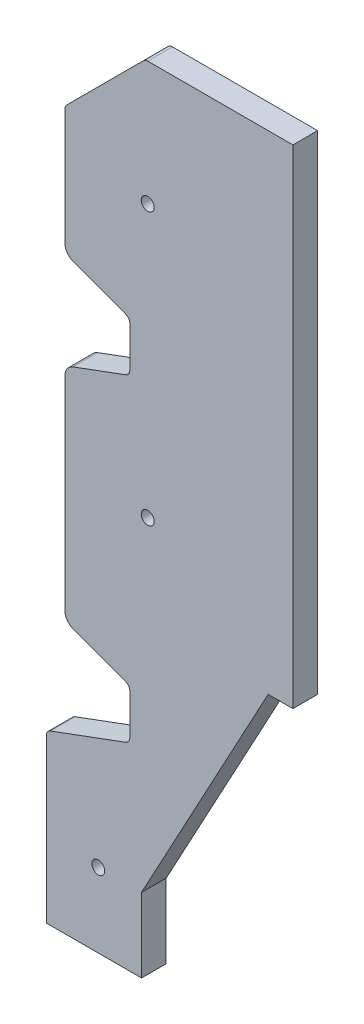
from build123d import *

# Parameters (mm, degrees)
BOSS_EXTRUDE1_DEPTH = 40
CHAMFER1_SIZE       = 160
M24_TAPPED_HOLE1_D  = 21
CUT_EXTRUDE1_DEPTH  = 1351.88896657
FILLET1_R           = 10
SKETCH4_W           = 30
SKETCH4_H           = 822.818816594
CUT_EXTRUDE2_DEPTH  = 1351.88896657
FILLET2_R           = 20
FILLET3_R           = 10


with BuildPart() as part:
    # Sketch1 → Boss-Extrude1 (new body)
    with BuildSketch(Plane.XY):
        Polygon((154, 0), (154, 120), (359, 500), (399, 500), (399, 1290), (0, 1290), (0, 0), align=None)
    extrude(amount=BOSS_EXTRUDE1_DEPTH)

    # Chamfer1
    chamfer1_edges = [part.edges().sort_by_distance(p)[0] for p in [
        (0, 1290, 20),
    ]]
    chamfer(chamfer1_edges, length=CHAMFER1_SIZE)

    # M24 Tapped Hole1 (through all)
    with Locations(Plane(origin=(164, 1090, 0), x_dir=(-1, 0, 0), z_dir=(0, 0, -1))):
        with Locations((0, 0), (0, -440), (80, -970)):
            Hole(M24_TAPPED_HOLE1_D / 2)

    # Sketch3 → Cut-Extrude1 (cut, through all)
    with BuildSketch(Plane(origin=(0, 0, 0), x_dir=(-1, 0, 0), z_dir=(0, 0, -1))):
        Polygon((-135, 835), (0, 785), (0, 965), (-135, 915), align=None)
        Polygon((-135, 400), (-135, 320), (0, 270), (0, 450), align=None)
    extrude(amount=-CUT_EXTRUDE1_DEPTH, mode=Mode.SUBTRACT)

    # Fillet1
    fillet1_edges = [part.edges().sort_by_distance(p)[0] for p in [
        (135, 400, 20),
        (0, 450, 20),
        (0, 270, 20),
        (135, 320, 20),
        (0, 965, 20),
        (0, 785, 20),
        (135, 835, 20),
        (135, 915, 20),
    ]]
    fillet(fillet1_edges, radius=FILLET1_R)

    # Sketch4 → Cut-Extrude2 (cut, through all)
    with BuildSketch(Plane(origin=(0, 0, 0), x_dir=(-1, 0, 0), z_dir=(0, 0, -1))):
        with Locations((-15, 748.590591703)):
            Rectangle(SKETCH4_W, SKETCH4_H)
    extrude(amount=-CUT_EXTRUDE2_DEPTH, mode=Mode.SUBTRACT)

    # Fillet2
    fillet2_edges = [part.edges().sort_by_distance(p)[0] for p in [
        (30, 953.888888889, 20),
        (30, 438.888888889, 20),
        (30, 796.111111111, 20),
    ]]
    fillet(fillet2_edges, radius=FILLET2_R)

    # Fillet3
    fillet3_edges = [part.edges().sort_by_distance(p)[0] for p in [
        (30, 1160, 20),
        (160, 1290, 20),
    ]]
    fillet(fillet3_edges, radius=FILLET3_R)


solid = part.part
